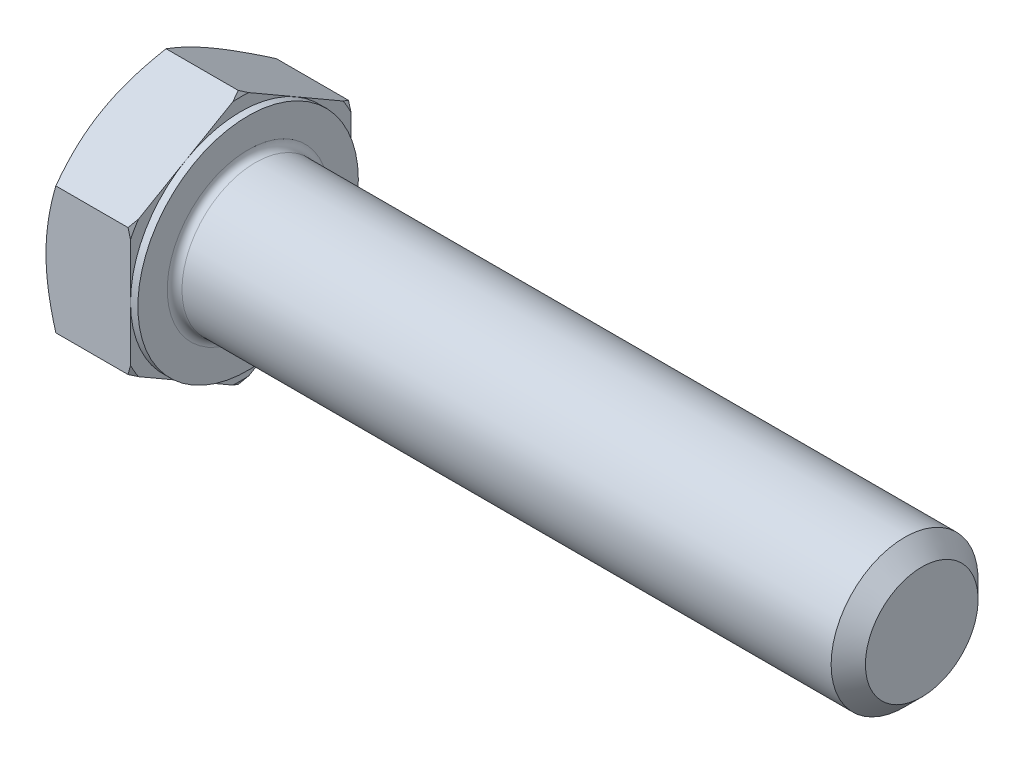
from build123d import *

# Parameters (mm, degrees)
BASE_EXTRUDE_DEPTH = 7.5
SKETCH4_W          = 0.6
SKETCH4_H          = 11.392304845
CHAMFER_2_SIZE     = 1.4
FILLET_2_R         = 0.6


with BuildPart() as part:
    # Sketch1 → Base-Extrude (new body)
    with BuildSketch(Plane(origin=(0, 0, 0), x_dir=(0, 0, -1), z_dir=(1, 0, 0))):
        Polygon((9, 5.196152423), (9, -5.196152423), (0, -10.392304845), (-9, -5.196152423), (-9, 5.196152423), (0, 10.392304845), align=None)
    extrude(amount=BASE_EXTRUDE_DEPTH)

    # Sketch2 → Boss-Revolve1 (revolve)
    with BuildSketch(Plane.XY, mode=Mode.PRIVATE) as boss_revolve1_sk:
        Polygon((0, 0), (62.5, 0), (62.5, 4.4845), (62.5, 6), (7.791693541, 6), (0, 6), align=None)
    revolve(boss_revolve1_sk.sketch.rotate(Axis((0, 0, 0), (1, 0, 0)), 90), axis=Axis((0, 0, 0), (1, 0, 0)))

    # Sketch3 → Cut-Revolve1 (revolve, cut)
    with BuildSketch(Plane.XY):
        Polygon((0, 9), (3.690598923, 15.392304845), (3.690598923, 20.392304845), (-10, 20.392304845), (-10, 9), align=None)
    revolve(axis=Axis((0, 0, 0), (1, 0, 0)), mode=Mode.SUBTRACT)

    # Sketch5 → Cut-Revolve2 (revolve, cut)
    with BuildSketch(Plane.XY):
        Polygon((7.5, 9), (3.809401077, 15.392304845), (3.809401077, 20.392304845), (13.809401077, 20.392304845), (13.809401077, 9), align=None)
    revolve(axis=Axis((0, 0, 0), (1, 0, 0)), mode=Mode.SUBTRACT)

    # Sketch4 → Cut-Revolve3 (revolve, cut)
    with BuildSketch(Plane.XY, mode=Mode.PRIVATE) as cut_revolve3_sk:
        with Locations((7.2, 14.696152423)):
            Rectangle(SKETCH4_W, SKETCH4_H)
    revolve(cut_revolve3_sk.sketch.rotate(Axis((0, 0, 0), (1, 0, 0)), 270), axis=Axis((0, 0, 0), (1, 0, 0)), mode=Mode.SUBTRACT)

    # Chamfer 2
    chamfer_2_edges = [part.edges().sort_by_distance(p)[0] for p in [
        (62.5, 0, -6),
    ]]
    chamfer(chamfer_2_edges, length=CHAMFER_2_SIZE)

    # Fillet 2
    fillet_2_edges = [part.edges().sort_by_distance(p)[0] for p in [
        (7.5, 0, -6),
    ]]
    fillet(fillet_2_edges, radius=FILLET_2_R)


solid = part.part
